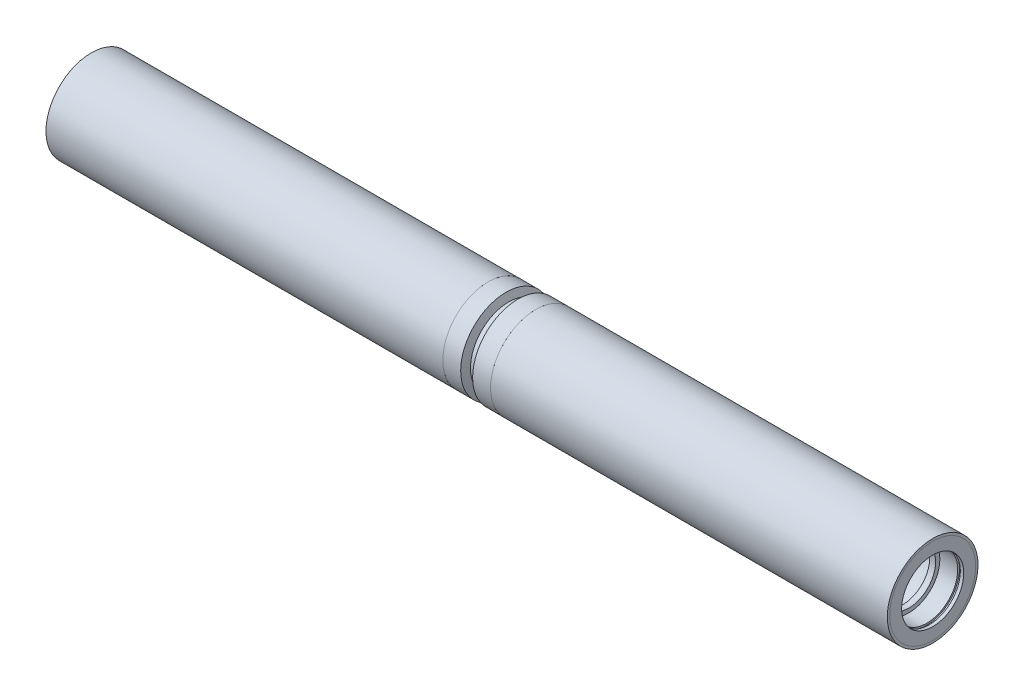
SolidWorks part; units mm, degrees
material "普通碳钢"
ref_plane "前视基准面" through (0, 0, 0) normal (0, 0, 1) x (1, 0, 0)
ref_plane "上视基准面" through (0, 0, 0) normal (0, 1, 0) x (1, 0, 0)
ref_plane "右视基准面" through (0, 0, 0) normal (1, 0, 0) x (0, 0, -1)
sketch "草图1" plane through (0, 0, 0) normal (0, 0, 1) x (1, 0, 0)
  line L0 (0, 0) -> (-250, 0) construction
  line L1 (0, 0) -> (0, 38) construction
  line L2 (-352.5, 36) -> (-352.5, 38)
  line L3 (352.5, 36) -> (352.5, 38)
  line L4 (0, 0) -> (250, 0) construction
  line L5 (-352.5, 36) -> (352.5, 36)
  line L6 (352.5, 38) -> (-352.5, 38)
  dimension "D1" = 76
  dimension "D2" = 2
  dimension "D3" = 705
revolve "旋转1" add sketch "草图1" angle 360 about L0
sketch "草图2" plane through (-352.5, 0, 0) normal (-1, 0, 0) x (0, 0, 1)
  circle A0 centre (0, 0) radius 36 construction
  circle A1 centre (0, 0) radius 36
  circle A2 centre (0, 0) radius 22.5
  dimension "D1" = 45
extrude "凸台-拉伸1" add sketch "草图2" against normal blind 25 separate body
sketch "草图3" plane through (352.5, 0, 0) normal (1, 0, 0) x (0, 0, -1)
  circle A1 centre (0, 0) radius 22.5
  circle A2 centre (0, 0) radius 22.5
  circle A3 centre (0, 0) radius 36
  circle A4 centre (0, 0) radius 36
  dimension "D1" = 0
  dimension "D2" = 0
extrude "凸台-拉伸2" add sketch "草图3" against normal blind 25 separate body
sketch "草图5" plane through (0, 0, 0) normal (0, 0, 1) x (1, 0, 0)
  line L8 (0, 0) -> (0, 70.2304) construction
  line L11 (0, 0) -> (-260.4475, 0) construction
  line L21 (-352.5, 26) -> (-349.7, 26)
  line L22 (-352.5, 38) -> (-352.5, -38) construction
  line L23 (-349.7, 26) -> (-349.7, 27.5)
  line L24 (-349.7, 27.5) -> (-347.5, 27.5)
  line L25 (-347.5, 27.5) -> (-347.5, 26)
  line L26 (-347.5, 26) -> (-332.5, 26)
  line L27 (-332.5, 26) -> (-332.5, 0)
  line L28 (-332.5, 0) -> (-352.5, 0)
  line L29 (-352.5, 0) -> (-352.5, 26)
  dimension "D1" = 52
  dimension "D2" = 55
  dimension "D3" = 2.2
  dimension "D4" = 2.8
  dimension "D5" = 20
  dimension "D6" = 15
revolve "切除-旋转6" cut sketch "草图5" angle 360 about L11
mirror "镜向2" about plane through (0, 0, 0) normal (1, 0, 0) of "切除-旋转6"
sketch "草图8" plane through (0, 0, 0) normal (0, 0, 1) x (1, 0, 0)
  line L1 (-20, 75.7733) -> (20, 75.7733)
  line L2 (-20, 75.7733) -> (-20, -75.7733)
  line L3 (-20, -75.7733) -> (20, -75.7733)
  line L4 (20, 75.7733) -> (20, -75.7733)
  line L5 (-20, 75.7733) -> (20, -75.7733) construction
  line L6 (-20, -75.7733) -> (20, 75.7733) construction
  point P0 (0, 0)
  dimension "D1" = 40
extrude "切除-拉伸1" cut sketch "草图8" against normal through all both and the other way through all
sketch "草图7" plane through (0, 0, 0) normal (0, 0, 1) x (1, 0, 0)
  line L0 (0, 0) -> (0, -63.5289) construction
  line L1 (-30, -36) -> (-20, -36)
  line L2 (0, 0) -> (49.1533, 0) construction
  line L3 (-20, -36) -> (-20, -38)
  line L4 (-20, -38) -> (20, -38)
  line L5 (-30, -36) -> (-30, -11)
  line L6 (-30, -11) -> (30, -11)
  line L7 (30, -36) -> (30, -11)
  line L8 (20, -36) -> (20, -38)
  line L9 (30, -36) -> (20, -36)
  line L10 (0, 0) -> (0, 37.0357) construction
  point P14 (0, -11)
  point P16 (0, -38)
  dimension "D1" = 40
  dimension "D2" = 60
  dimension "D3" = 11
  dimension "D4" = 2
  dimension "D5" = 38
revolve "旋转2" add sketch "草图7" angle 360 about L2
sketch "草图6" plane through (0, 0, 0) normal (0, 0, 1) x (1, 0, 0)
  line L6 (0, 0) -> (0, 115.6759) construction
  line L7 (-2.8162, 32) -> (2.8162, 32)
  line L13 (0, 0) -> (-158.4265, 0) construction
  line L14 (-5, 38) -> (-2.8162, 32)
  line L15 (5, 38) -> (2.8162, 32)
  line L16 (-5, 38) -> (5, 38)
  point P25 (0, 32)
  dimension "D5" = 10
  dimension "D6" = 6
  dimension "D7" = 40
revolve "切除-旋转7" cut sketch "草图6" angle 360 about L13
